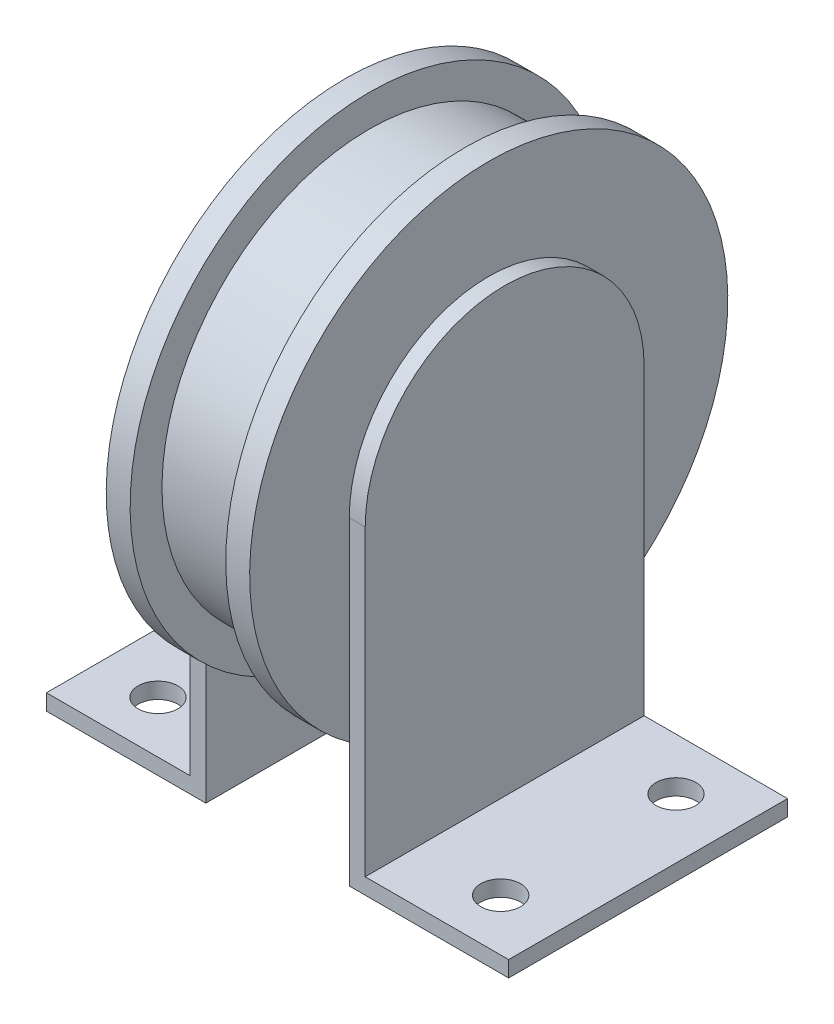
from build123d import *

# Parameters (mm, degrees)
EXTRUDE_1_DEPTH     = 2
SKETCH_3_W          = 35
SKETCH_3_H          = 2
EXTRUDE_2_DEPTH     = 18
CUT_EXTRUDE_1_REACH = 87.112
SKETCH_4_R          = 2.5


with BuildPart() as part:
    # 草图1 → 旋转1 (revolve)
    with BuildSketch(Plane.XY):
        Polygon((0, 30), (0, 18.550632587), (0, 0), (18, 0), (18, 30), (15, 30), (15, 26), (3, 26), (3, 30), align=None)
    revolve(axis=Axis((18, 0, 0), (-1, 0, 0)))

    # 草图2 → 凸台-拉伸1 (add)
    with BuildSketch(Plane(origin=(18, 0, 0), x_dir=(0, 0, -1), z_dir=(1, 0, 0))):
        with BuildLine():
            Line((17.5, -40), (17.5, 0))
            ThreePointArc((17.5, 0), (0, 17.5), (-17.5, 0))
            Line((-17.5, 0), (-17.5, -40))
            Line((-17.5, -40), (17.5, -40))
        make_face()
    extrude_1 = extrude(amount=EXTRUDE_1_DEPTH)

    # 草图3 → 凸台-拉伸2 (add)
    with BuildSketch(Plane(origin=(20, 0, 0), x_dir=(0, 0, -1), z_dir=(1, 0, 0))):
        with Locations((0, -39)):
            Rectangle(SKETCH_3_W, SKETCH_3_H)
    extrude_2 = extrude(amount=EXTRUDE_2_DEPTH)

    # 镜向1: 凸台-拉伸1, 凸台-拉伸2 across plane
    add(extrude_1.mirror(Plane(origin=(9, 0, 0), x_dir=(0, 0, 1), z_dir=(1, 0, 0))))
    add(extrude_2.mirror(Plane(origin=(9, 0, 0), x_dir=(0, 0, 1), z_dir=(1, 0, 0))))

    # 草图4 → 切除-拉伸1 (cut, up to next)
    with BuildSketch(Plane.XZ.offset(40), mode=Mode.PRIVATE) as cut_extrude_1_sk1:
        with Locations((-12.5, 11)):
            Circle(SKETCH_4_R)
    cut_extrude_1_tool1 = extrude(cut_extrude_1_sk1.sketch, amount=-CUT_EXTRUDE_1_REACH, mode=Mode.PRIVATE) & part.part
    # 草图4 → 切除-拉伸1 (cut, up to next)
    with BuildSketch(Plane.XZ.offset(40), mode=Mode.PRIVATE) as cut_extrude_1_sk2:
        with Locations(Location((-12.5, -11, 0), (0, 0, 180))):
            Circle(SKETCH_4_R)
    cut_extrude_1_tool2 = extrude(cut_extrude_1_sk2.sketch, amount=-CUT_EXTRUDE_1_REACH, mode=Mode.PRIVATE) & part.part
    # 草图4 → 切除-拉伸1 (cut, up to next)
    with BuildSketch(Plane.XZ.offset(40), mode=Mode.PRIVATE) as cut_extrude_1_sk3:
        with Locations((30.5, -11)):
            Circle(SKETCH_4_R)
    cut_extrude_1_tool3 = extrude(cut_extrude_1_sk3.sketch, amount=-CUT_EXTRUDE_1_REACH, mode=Mode.PRIVATE) & part.part
    # 草图4 → 切除-拉伸1 (cut, up to next)
    with BuildSketch(Plane.XZ.offset(40), mode=Mode.PRIVATE) as cut_extrude_1_sk4:
        with Locations((30.5, 11)):
            Circle(SKETCH_4_R)
    cut_extrude_1_tool4 = extrude(cut_extrude_1_sk4.sketch, amount=-CUT_EXTRUDE_1_REACH, mode=Mode.PRIVATE) & part.part
    add(cut_extrude_1_tool1.solids().sort_by_distance((-12.5, -40, 11))[0], mode=Mode.SUBTRACT)
    add(cut_extrude_1_tool2.solids().sort_by_distance((-12.5, -40, -11))[0], mode=Mode.SUBTRACT)
    add(cut_extrude_1_tool3.solids().sort_by_distance((30.5, -40, -11))[0], mode=Mode.SUBTRACT)
    add(cut_extrude_1_tool4.solids().sort_by_distance((30.5, -40, 11))[0], mode=Mode.SUBTRACT)


solid = part.part
